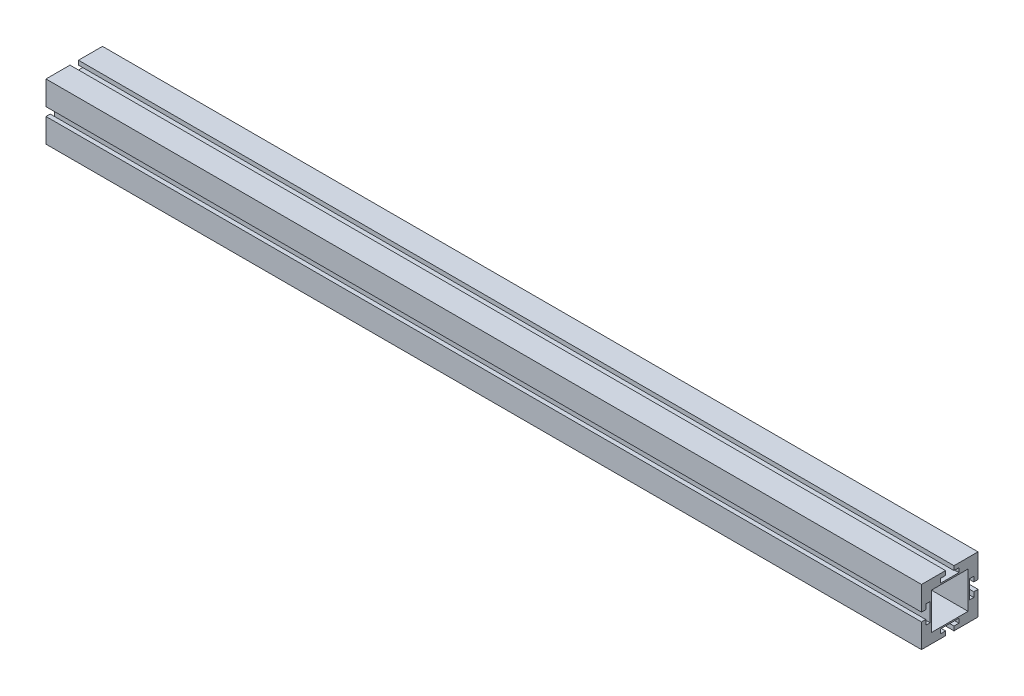
SolidWorks part; units mm, degrees
ref_plane "Front Plane" through (0, 0, 0) normal (0, 0, 1) x (1, 0, 0)
ref_plane "Top Plane" through (0, 0, 0) normal (0, 1, 0) x (1, 0, 0)
ref_plane "Right Plane" through (0, 0, 0) normal (1, 0, 0) x (0, 0, -1)
sketch "Sketch1" plane through (0, 0, 0) normal (1, 0, 0) x (0, 0, -1)
  line L0 (0, 0) -> (0, 33.8923) construction
  line L1 (-20, -20) -> (-3, -20)
  line L2 (-20, -20) -> (-20, -3)
  line L3 (-20, 20) -> (-3, 20)
  line L4 (20, -20) -> (20, -3)
  line L5 (-20, -20) -> (20, 20) construction
  line L6 (-20, 20) -> (20, -20) construction
  line L7 (-13, -13) -> (13, -13)
  line L8 (-13, -13) -> (-13, 13)
  line L9 (-13, 13) -> (13, 13)
  line L10 (13, -13) -> (13, 13)
  line L11 (-13, -13) -> (13, 13) construction
  line L12 (-13, 13) -> (13, -13) construction
  line L13 (0, 0) -> (25.505, 0) construction
  line L14 (17, 3) -> (17, 6.5)
  line L15 (-6.5, 17) -> (-3, 17)
  line L16 (6.5, 17) -> (6.5, 14)
  line L17 (3, 17) -> (6.5, 17)
  line L18 (-6.5, 14) -> (6.5, 14)
  line L19 (17, -6.5) -> (17, -3)
  line L20 (3, 20) -> (20, 20)
  line L21 (14, -6.5) -> (17, -6.5)
  line L22 (-3, 20) -> (-3, 17)
  line L23 (17, 3) -> (20, 3)
  line L24 (3, 20) -> (3, 17)
  line L25 (17, -3) -> (20, -3)
  line L26 (-20, 20) -> (20, 20) construction
  line L27 (14, -6.5) -> (14, 6.5)
  line L28 (-17, -17) -> (17, -17) construction
  line L29 (20, 3) -> (20, 20)
  line L30 (-6.5, 17) -> (-6.5, 14)
  line L31 (14, 6.5) -> (17, 6.5)
  line L32 (14, -14) -> (14, 14) construction
  line L33 (-14, 14) -> (14, 14) construction
  line L34 (-17, 17) -> (17, 17) construction
  line L35 (3, -20) -> (3, -17)
  line L36 (-17, -17) -> (-17, 17) construction
  line L37 (-14, -14) -> (-14, 14) construction
  line L38 (-14, -14) -> (14, -14) construction
  line L39 (17, -17) -> (17, 17) construction
  line L40 (20, -20) -> (20, 20) construction
  line L41 (3, -17) -> (6.5, -17)
  line L42 (6.5, -17) -> (6.5, -14)
  line L43 (-6.5, -14) -> (6.5, -14)
  line L44 (-6.5, -17) -> (-6.5, -14)
  line L45 (-6.5, -17) -> (-3, -17)
  line L46 (-3, -20) -> (-3, -17)
  line L47 (-14, -6.5) -> (-14, 6.5)
  line L48 (-14, -6.5) -> (-17, -6.5)
  line L49 (-17, -6.5) -> (-17, -3)
  line L50 (-17, -3) -> (-20, -3)
  line L51 (-17, 3) -> (-20, 3)
  line L52 (-17, 3) -> (-17, 6.5)
  line L53 (-14, 6.5) -> (-17, 6.5)
  line L54 (-20, 3) -> (-20, 20)
  line L55 (3, -20) -> (20, -20)
  line L56 (-20, -20) -> (-20, 20) construction
  line L58 (-20, -20) -> (20, -20) construction
  point P0 (0, 0)
  point P6 (0, 0)
  dimension "D1" = 40
  dimension "D2" = 40
  dimension "D3" = 26
  dimension "D4" = 26
  dimension "D7" = 3
  dimension "D8" = 3
  dimension "D9" = 6
  dimension "D10" = 13
  dimension "D11" = 3
  dimension "D12" = 6
  dimension "D13" = 13
  dimension "D5" = 3
  dimension "D6" = 3
extrude "Boss-Extrude1" add sketch "Sketch1" along normal blind 620
